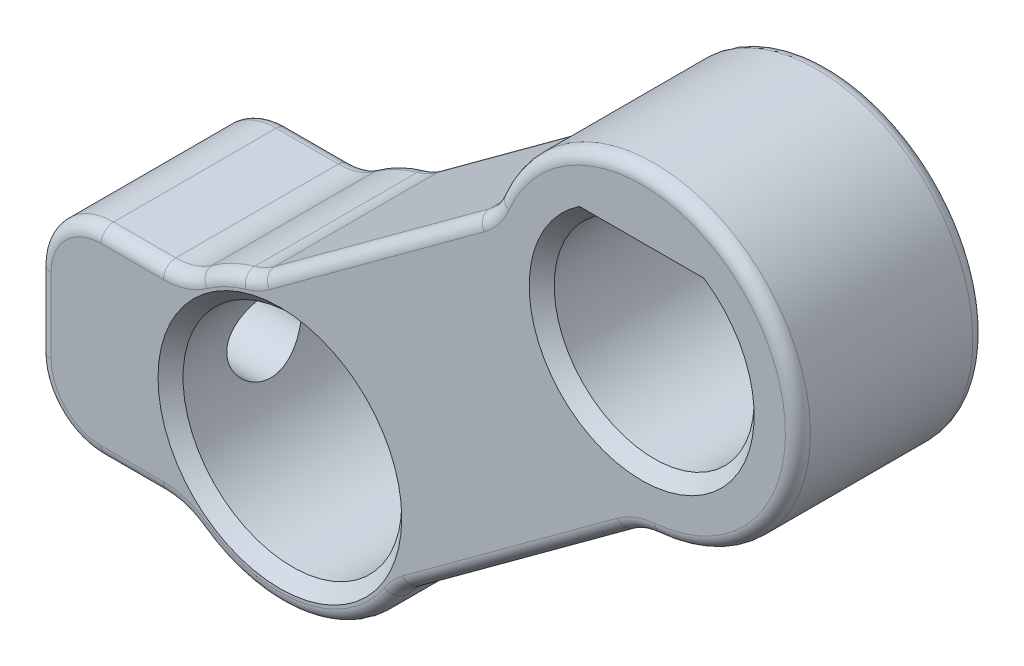
SolidWorks part; units mm, degrees
ref_plane "前视基准面" through (0, 0, 0) normal (0, 0, 1) x (1, 0, 0)
ref_plane "上视基准面" through (0, 0, 0) normal (0, 1, 0) x (1, 0, 0)
ref_plane "右视基准面" through (0, 0, 0) normal (1, 0, 0) x (0, 0, -1)
sketch "草图1" plane through (0, 0, 0) normal (0, 0, 1) x (1, 0, 0)
  line L1 (-294.9933, -10.0695) -> (-276.3386, -10.0695)
  line L2 (-285.666, -23.0695) -> (-343.5594, -65.5012) construction
  line L3 (-309.5874, -15.8055) -> (-347.9901, -43.952)
  line L4 (-285.9413, -48.068) -> (-324.3441, -76.2144)
  line L5 (-297.489, -6.9383) -> (-355.3824, -49.37) construction
  line L6 (-273.8429, -39.2007) -> (-331.7363, -81.6324) construction
  line L7 (-343.5594, -65.5012) -> (-382.1594, -65.5012) construction
  line L8 (-358.659, -49.5012) -> (-382.1594, -49.5012)
  line L9 (-358.659, -81.5012) -> (-382.1594, -81.5012)
  line L10 (-343.5594, -65.5012) -> (-391.9275, -65.5012) construction
  line L11 (-382.1594, -65.5012) -> (-382.1594, -49.5012)
  line L12 (-382.1594, -65.5012) -> (-382.1594, -81.5012)
  line L13 (-343.5594, -49.5012) -> (-391.9275, -49.5012) construction
  line L14 (-343.5594, -81.5012) -> (-391.9275, -81.5012) construction
  circle A1 centre (-343.5594, -65.5012) radius 17.5
  circle A2 centre (-285.666, -23.0695) radius 21.75 construction
  arc A3 (-294.9933, -10.0695) -> (-276.3386, -10.0695) centre (-285.666, -23.0695) ccw
  arc A4 (-347.9901, -43.952) -> (-358.659, -49.5012) centre (-343.5594, -65.5012) ccw
  arc A5 (-285.9413, -48.068) -> (-309.5874, -15.8055) centre (-285.666, -23.0695) ccw
  arc A6 (-358.659, -81.5012) -> (-324.3441, -76.2144) centre (-343.5594, -65.5012) ccw
extrude "凸台-拉伸1" add sketch "草图1" along normal blind 30
fillet "圆角1" radius 10 8 edges at (-347.9901, -43.952, 15) (-309.5874, -15.8055, 15) (-324.3441, -76.2144, 15) (-358.659, -81.5012, 15) (-382.1594, -81.5012, 15) (-382.1594, -49.5012, 15) (-358.659, -49.5012, 15) (-285.9413, -48.068, 15)
fillet "圆角2" radius 2 32 edges at (-310.0889, -15.7221, 0) (-265.502, -8.2907, 0) (-286.0128, -48.5713, 0) (-305.5691, -62.4537, 0) (-324.0876, -76.2217, 0) (-339.5608, -87.1348, 0) (-359.1523, -81.9815, 0) (-367.1867, -81.5012, 0) (-379.2304, -78.5723, 0) (-382.1594, -65.5012, 0) (-379.2304, -52.4301, 0) (-367.1867, -49.5012, 0) (-359.1523, -49.0209, 0) (-353.123, -45.6887, 0) (-347.9198, -43.7052, 0) (-310.0889, -15.7221, 30) (-265.502, -8.2907, 30) (-286.0128, -48.5713, 30) (-305.5691, -62.4537, 30) (-324.0876, -76.2217, 30) (-339.5608, -87.1348, 30) (-359.1523, -81.9815, 30) (-367.1867, -81.5012, 30) (-379.2304, -78.5723, 30) (-382.1594, -65.5012, 30) (-379.2304, -52.4301, 30) (-367.1867, -49.5012, 30) (-359.1523, -49.0209, 30) (-353.123, -45.6887, 30) (-347.9198, -43.7052, 30) (-329.2152, -30.1913, 0) (-329.2152, -30.1913, 30)
chamfer "倒角1" distance 2 angle 45 6 edges at (-285.666, -10.0695, 0) (-285.666, -39.0695, 0) (-285.666, -10.0695, 30) (-285.666, -39.0695, 30) (-326.0594, -65.5012, 0) (-326.0594, -65.5012, 30)
sketch "草图2" plane through (-382.1594, 0, 0) normal (-1, 0, 0) x (0, 0, 1)
  line L0 (2, -59.5012) -> (2, -71.5012) construction
  line L1 (28, -59.5012) -> (2, -59.5012) construction
  circle A0 centre (15, -65.5012) radius 6
  point P4 (2, -65.5012)
  point P7 (15, -59.5012)
  dimension "D1" = 12
extrude "切除-拉伸1" cut sketch "草图2" against normal blind 50
equation "\"D2@草图1\"=\"D1@草图1\""
equation "\"D4@草图1\"=\"D3@草图1\""
